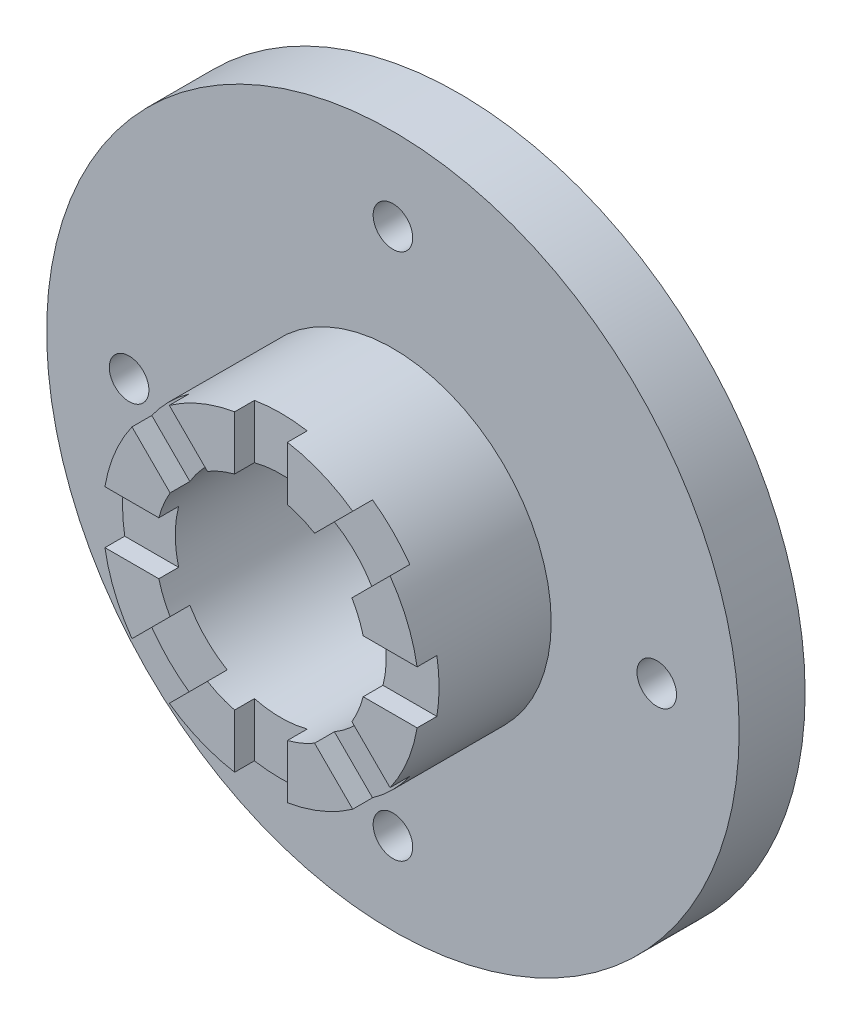
SolidWorks part; units mm, degrees
ref_plane "前视基准面" through (0, 0, 0) normal (0, 0, 1) x (1, 0, 0)
ref_plane "上视基准面" through (0, 0, 0) normal (0, 1, 0) x (1, 0, 0)
ref_plane "右视基准面" through (0, 0, 0) normal (1, 0, 0) x (0, 0, -1)
sketch "草图1" plane through (0, 0, 0) normal (0, 0, 1) x (1, 0, 0)
  circle A0 centre (0, 0) radius 52.5
  circle A1 centre (0, 0) radius 24
  circle A2 centre (0, 0) radius 16
  circle A3 centre (0, 0) radius 40 construction
  circle A4 centre (0, 40) radius 3
  circle A5 centre (40, 0) radius 3
  circle A6 centre (0, -40) radius 3
  circle A7 centre (-40, 0) radius 3
  dimension "D1" = 105
  dimension "D2" = 48
  dimension "D3" = 32
  dimension "D4" = 80
  dimension "D5" = 6
  dimension "D6" = 4
extrude "凸台-拉伸1" add sketch "草图1" along normal blind 10 contours A0 A1 | A1 A2
cosmetic thread "装饰螺纹线1" parameters "D2"=36
sketch "草图2" plane through (0, 0, 10) normal (0, 0, 1) x (1, 0, 0)
  circle A0 centre (0, 0) radius 16 construction
  circle A1 centre (0, 0) radius 16
  circle A2 centre (0, 0) radius 24 construction
  circle A3 centre (0, 0) radius 24
extrude "凸台-拉伸2" add sketch "草图2" along normal blind 20
sketch "草图3" plane through (0, 0, 30) normal (0, 0, 1) x (1, 0, 0)
  line L0 (0, 24) -> (0, 16) construction
  line L1 (-4, 23.6643) -> (-4, 15.4919)
  line L2 (4, 23.6643) -> (4, 15.4919)
  line L3 (13.9048, 19.5616) -> (8.126, 13.7829)
  line L4 (19.5616, 13.9048) -> (13.7829, 8.126)
  line L5 (23.6643, 4) -> (15.4919, 4)
  line L6 (23.6643, -4) -> (15.4919, -4)
  line L7 (19.5616, -13.9048) -> (13.7829, -8.126)
  line L8 (13.9048, -19.5616) -> (8.126, -13.7829)
  line L9 (4, -23.6643) -> (4, -15.4919)
  line L10 (-4, -23.6643) -> (-4, -15.4919)
  line L11 (-13.9048, -19.5616) -> (-8.126, -13.7829)
  line L12 (-19.5616, -13.9048) -> (-13.7829, -8.126)
  line L13 (-23.6643, -4) -> (-15.4919, -4)
  line L14 (-23.6643, 4) -> (-15.4919, 4)
  line L15 (-19.5616, 13.9048) -> (-13.7829, 8.126)
  line L16 (-13.9048, 19.5616) -> (-8.126, 13.7829)
  circle A0 centre (0, 0) radius 24 construction
  arc A1 (4, 23.6643) -> (-4, 23.6643) centre (0, 0) ccw
  circle A2 centre (0, 0) radius 16 construction
  arc A3 (4, 15.4919) -> (-4, 15.4919) centre (0, 0) ccw
  arc A4 (19.5616, 13.9048) -> (13.9048, 19.5616) centre (0, 0) ccw
  arc A5 (13.7829, 8.126) -> (8.126, 13.7829) centre (0, 0) ccw
  arc A6 (23.6643, -4) -> (23.6643, 4) centre (0, 0) ccw
  arc A7 (15.4919, -4) -> (15.4919, 4) centre (0, 0) ccw
  arc A8 (8.126, -13.7829) -> (13.7829, -8.126) centre (0, 0) ccw
  arc A9 (13.9048, -19.5616) -> (19.5616, -13.9048) centre (0, 0) ccw
  arc A10 (-4, -23.6643) -> (4, -23.6643) centre (0, 0) ccw
  arc A11 (-4, -15.4919) -> (4, -15.4919) centre (0, 0) ccw
  arc A12 (-19.5616, -13.9048) -> (-13.9048, -19.5616) centre (0, 0) ccw
  arc A13 (-13.7829, -8.126) -> (-8.126, -13.7829) centre (0, 0) ccw
  arc A14 (-23.6643, 4) -> (-23.6643, -4) centre (0, 0) ccw
  arc A15 (-15.4919, 4) -> (-15.4919, -4) centre (0, 0) ccw
  arc A16 (-13.9048, 19.5616) -> (-19.5616, 13.9048) centre (0, 0) ccw
  arc A17 (-8.126, 13.7829) -> (-13.7829, 8.126) centre (0, 0) ccw
  dimension "D1" = 4
  dimension "D2" = 8
extrude "切除-拉伸2" cut sketch "草图3" against normal blind 3
